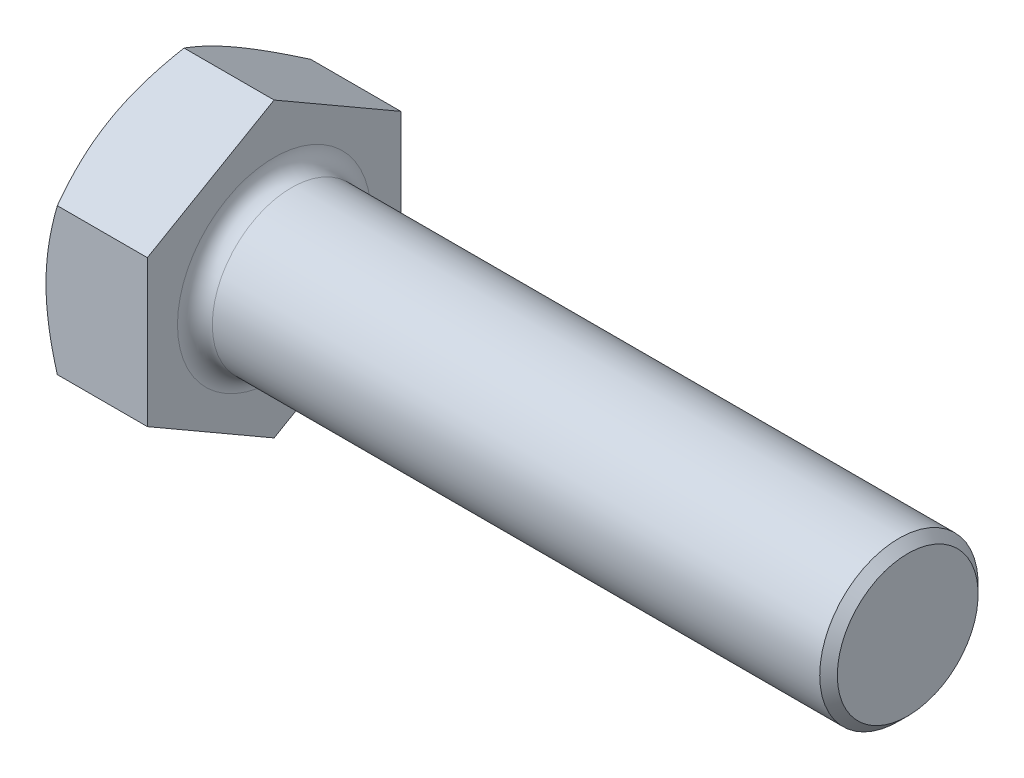
from build123d import *

# Parameters (mm, degrees)
BOSS_EXTRUDE1_DEPTH = 6.4
SKETCH4_R           = 17.59
SKETCH4_R_2         = 8
CUT_EXTRUDE1_DEPTH  = 0.8
CUT_EXTRUDE1_DRAFT  = -60
CHAMFER2_SIZE       = 0.555555556


with BuildPart() as part:
    # Sketch3 → Boss-Extrude1 (new body)
    with BuildSketch(Plane(origin=(0, 0, 0), x_dir=(0, 0, -1), z_dir=(1, 0, 0))):
        Polygon((8, 4.618802154), (0, 9.237604307), (-8, 4.618802154), (-8, -4.618802154), (0, -9.237604307), (8, -4.618802154), align=None)
    extrude(amount=BOSS_EXTRUDE1_DEPTH)


with BuildPart() as cut_extrude1_tool:
    # Sketch4 → Cut-Extrude1 (with draft: the straight prism first)
    with BuildSketch(Plane.ZY):
        Circle(SKETCH4_R)
        Circle(SKETCH4_R_2, mode=Mode.SUBTRACT)
    extrude(amount=-CUT_EXTRUDE1_DEPTH)
    # Cut-Extrude1: the draft: its side faces are tilted about the plane it starts from
    cut_extrude1_sides = [cut_extrude1_tool.faces().sort_by_distance(p)[0] for p in [
        (0.4, 0, -17.59),
        (0.4, 0, -8),
    ]]
    draft(cut_extrude1_sides, Plane.ZY, CUT_EXTRUDE1_DRAFT)


with BuildPart() as part_1:
    add(part.part)

    # Cut-Extrude1: cut by cut_extrude1_tool
    add(cut_extrude1_tool.part, mode=Mode.SUBTRACT)

    # Sketch5 → Revolve1 (revolve)
    with BuildSketch(Plane.XY, mode=Mode.PRIVATE) as revolve1_sk:
        with BuildLine():
            Line((7.5, 5), (46.4, 5))
            Line((46.4, 5), (46.4, 0))
            Line((46.4, 0), (6.4, 0))
            Line((6.4, 0), (6.4, 6.1))
            ThreePointArc((6.4, 6.1), (6.722182541, 5.322182541), (7.5, 5))
        make_face()
    revolve(revolve1_sk.sketch.rotate(Axis((6.4, 0, 0), (1, 0, 0)), 90), axis=Axis((6.4, 0, 0), (1, 0, 0)))

    # Chamfer2
    chamfer2_edges = [part_1.edges().sort_by_distance(p)[0] for p in [
        (46.4, 0, -5),
    ]]
    chamfer(chamfer2_edges, length=CHAMFER2_SIZE)


solid = part_1.part
